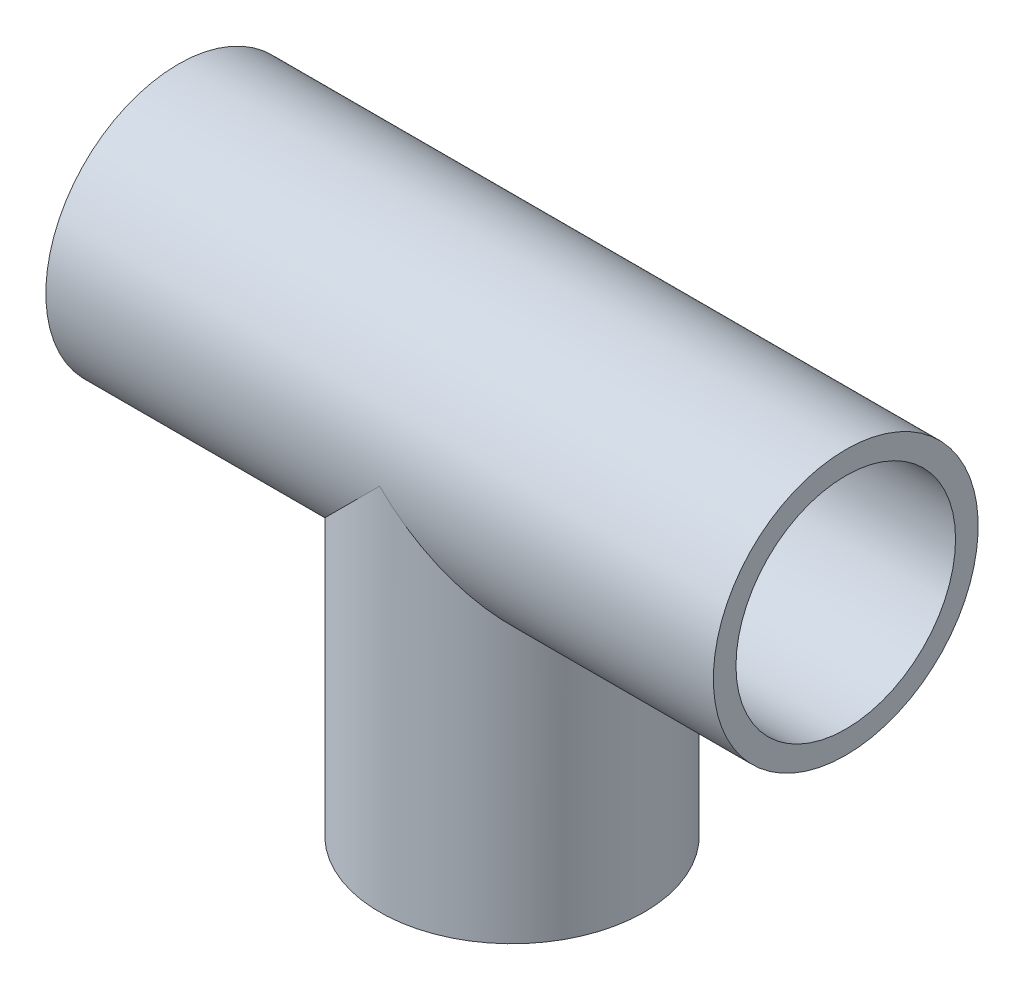
from build123d import *

# Parameters (mm, degrees)
SWEEP_THIN_PART_1_PROFILE_R   = 30.15
SWEEP_THIN_PART_1_PROFILE_R_2 = 25
SWEEP_THIN_PART_2_PROFILE_R   = 30.15
SWEEP_THIN_PART_2_PROFILE_R_2 = 25
SKETCH15_R                    = 25
CUT_EXTRUDE1_DEPTH            = 177.264070494
SKETCH18_R                    = 25
CUT_EXTRUDE2_DEPTH            = 85


with BuildPart() as part:
    # Sweep-thin part 1: sweep along a path in Sketch1
    with BuildLine(Plane.XY) as sweep_thin_part_1_path:
        Line((-76, 0), (76, 0))
    # Sweep-thin part 1 profile (on start of the path) → Sweep-thin part 1 (sweep)
    with BuildSketch(Plane.YZ.offset(-76)):
        Circle(SWEEP_THIN_PART_1_PROFILE_R)
        Circle(SWEEP_THIN_PART_1_PROFILE_R_2, mode=Mode.SUBTRACT)
    sweep(path=sweep_thin_part_1_path.line)

    # Sweep-thin part 2: sweep along a path in Sketch8
    with BuildLine(Plane.XY) as sweep_thin_part_2_path:
        Line((0, 0), (0, -84))
    # Sweep-thin part 2 profile (on start of the path) → Sweep-thin part 2 (sweep)
    with BuildSketch(Plane(origin=(0, 0, 0), x_dir=(-1, 0, 0), z_dir=(0, -1, 0))):
        Circle(SWEEP_THIN_PART_2_PROFILE_R)
        Circle(SWEEP_THIN_PART_2_PROFILE_R_2, mode=Mode.SUBTRACT)
    sweep(path=sweep_thin_part_2_path.line)

    # Sketch15 → Cut-Extrude1 (cut, through all)
    with BuildSketch(Plane.ZY.offset(76)):
        with Locations(Location((0, 0, 0), (0, 0, 90))):
            Circle(SKETCH15_R)
    extrude(amount=-CUT_EXTRUDE1_DEPTH, mode=Mode.SUBTRACT)

    # Sketch18 → Cut-Extrude2 (cut)
    with BuildSketch(Plane.XZ.offset(84)):
        Circle(SKETCH18_R)
    extrude(amount=-CUT_EXTRUDE2_DEPTH, mode=Mode.SUBTRACT)


solid = part.part
